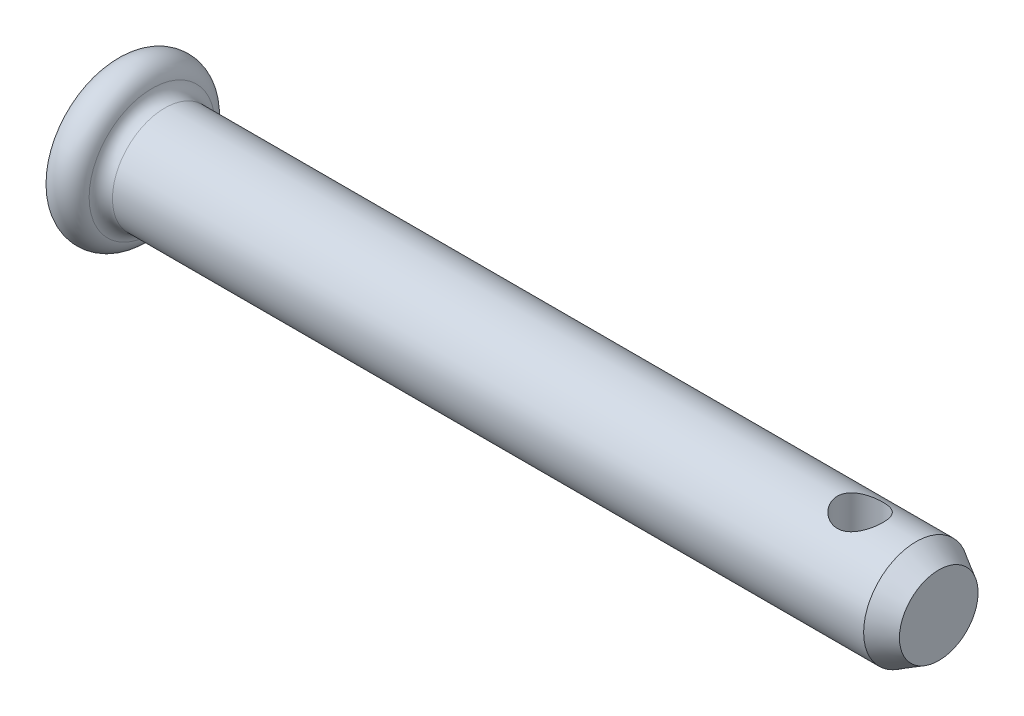
from build123d import *

# Parameters (mm, degrees)
FILLET_1_R          = 0.5
CHAMFER_1_SIZE      = 0.866025404
CHAMFER_1_SIZE2     = 0.5
SKETCH_2_R          = 0.87
CUT_EXTRUDE_1_DEPTH = 500


with BuildPart() as part:
    # 草图1 → Revolve 700 (revolve)
    with BuildSketch(Plane.XY, mode=Mode.PRIVATE) as revolve_700_sk:
        with BuildLine():
            Line((0, 0), (31.5, 0))
            Line((31.5, 0), (31.5, 2))
            Line((31.5, 2), (1.5, 2))
            Line((1.5, 2), (1.5, 2.25))
            ThreePointArc((1.5, 2.25), (0.75, 3), (0, 2.25))
            Line((0, 2.25), (0, 0))
        make_face()
    revolve(revolve_700_sk.sketch.rotate(Axis((0, 0, 0), (1, 0, 0)), 90), axis=Axis((0, 0, 0), (1, 0, 0)))

    # 圆角1
    fillet_1_edges = [part.edges().sort_by_distance(p)[0] for p in [
        (1.5, 0, -2),
    ]]
    fillet(fillet_1_edges, radius=FILLET_1_R)

    # 倒角1
    chamfer_1_edges = [part.edges().sort_by_distance(p)[0] for p in [
        (31.5, 0, -2),
    ]]
    chamfer_1_side = [part.faces().sort_by_distance(p)[0] for p in [
        (16.737372436, 0, -2),
    ]]
    chamfer(chamfer_1_edges, length=CHAMFER_1_SIZE, length2=CHAMFER_1_SIZE2, reference=chamfer_1_side[0])

    # 草图2 → 切除-拉伸1 (cut, symmetric)
    with BuildSketch(Plane(origin=(0, 0, 0), x_dir=(1, 0, 0), z_dir=(0, 1, 0))):
        with Locations(Location((28.5, 0, 0), (0, 0, 270))):
            Circle(SKETCH_2_R)
    extrude(amount=CUT_EXTRUDE_1_DEPTH, both=True, mode=Mode.SUBTRACT)


solid = part.part
